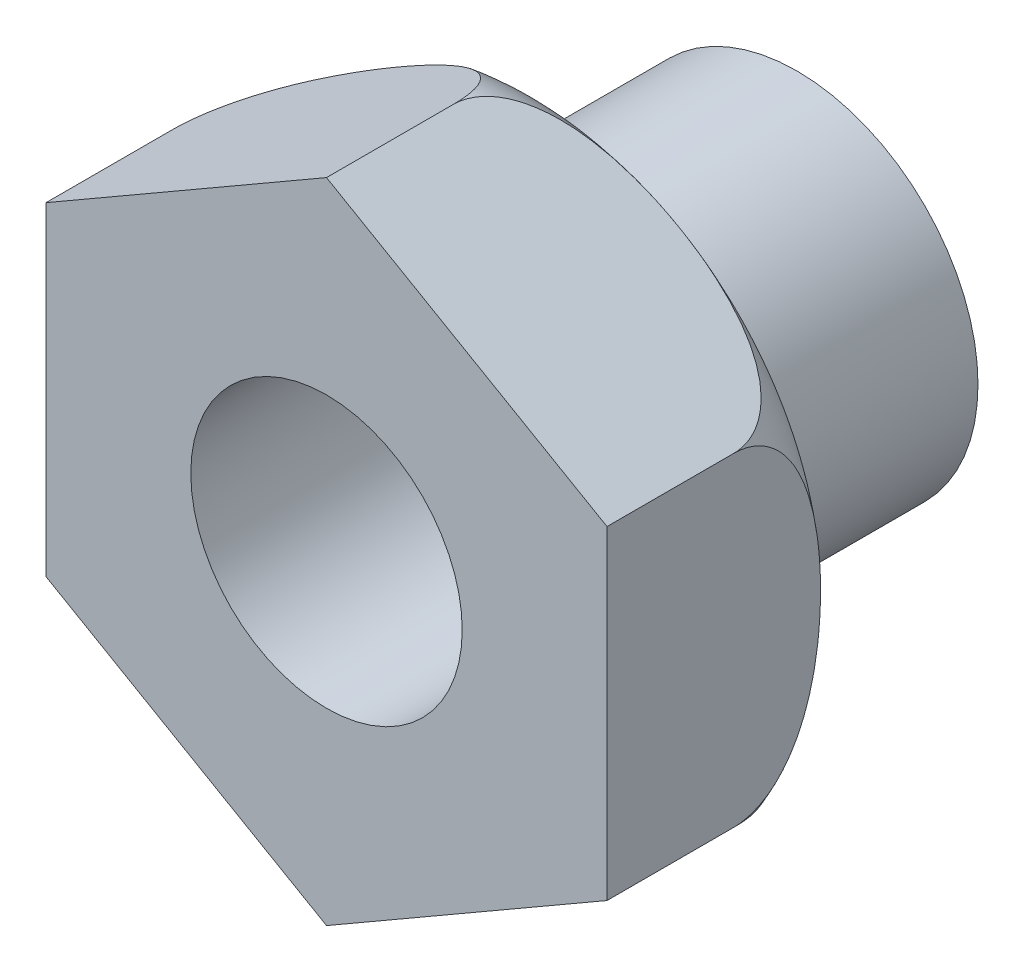
from build123d import *

# Parameters (mm, degrees)
BOSS_EXTRUDE1_DEPTH = 65
SKETCH3_R           = 50
SKETCH3_R_2         = 37.5
BOSS_EXTRUDE2_DEPTH = 65
SKETCH4_R           = 37.5
CUT_EXTRUDE2_DEPTH  = 130


with BuildPart() as part:
    # Sketch1 → Boss-Extrude1 (new body)
    with BuildSketch(Plane.XY):
        Polygon((77.5, 44.744645862), (0, 89.489291724), (-77.5, 44.744645862), (-77.5, -44.744645862), (0, -89.489291724), (77.5, -44.744645862), align=None)
    extrude(amount=BOSS_EXTRUDE1_DEPTH)

    # Sketch2 → Cut-Revolve1 (revolve, cut)
    with BuildSketch(Plane(origin=(0, 0, 0), x_dir=(0, 0, -1), z_dir=(1, 0, 0)), mode=Mode.PRIVATE) as cut_revolve1_sk:
        with BuildLine():
            Line((0, 59.489291724), (0, 89.489291724))
            Line((0, 89.489291724), (-30, 89.489291724))
            ThreePointArc((-30, 89.489291724), (-8.786796564, 80.70249516), (0, 59.489291724))
        make_face()
    revolve(cut_revolve1_sk.sketch.rotate(Axis((0, 0, 90.10395437), (0, 0, -1)), 90), axis=Axis((0, 0, 90.10395437), (0, 0, -1)), mode=Mode.SUBTRACT)

    # Sketch3 → Boss-Extrude2 (add)
    with BuildSketch(Plane(origin=(0, 0, 0), x_dir=(-1, 0, 0), z_dir=(0, 0, -1))):
        with Locations(Location((0, 0, 0), (0, 0, 180))):
            Circle(SKETCH3_R)
        Circle(SKETCH3_R_2, mode=Mode.SUBTRACT)
    extrude(amount=BOSS_EXTRUDE2_DEPTH)

    # Sketch4 → Cut-Extrude2 (cut)
    with BuildSketch(Plane.XY.offset(65)):
        Circle(SKETCH4_R)
    extrude(amount=-CUT_EXTRUDE2_DEPTH, mode=Mode.SUBTRACT)


solid = part.part
